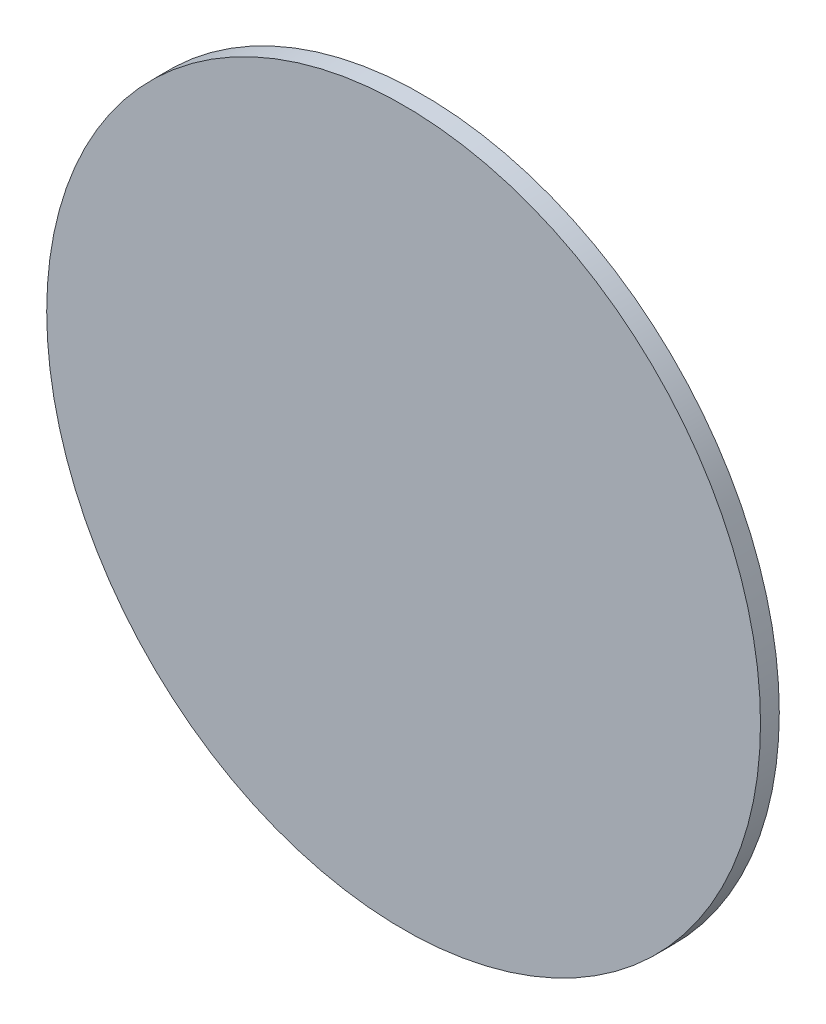
SolidWorks part; units mm, degrees
ref_plane "Front Plane" through (0, 0, 0) normal (0, 0, 1) x (1, 0, 0)
ref_plane "Top Plane" through (0, 0, 0) normal (0, 1, 0) x (1, 0, 0)
ref_plane "Right Plane" through (0, 0, 0) normal (1, 0, 0) x (0, 0, -1)
other "Configuration Table"
sketch "Sketch1" plane through (0, 0, 0) normal (0, 0, 1) x (1, 0, 0)
  circle A0 centre (0, 0) radius 380
  dimension "D1" = 760
extrude "Boss-Extrude1" add sketch "Sketch1" along normal blind 20
